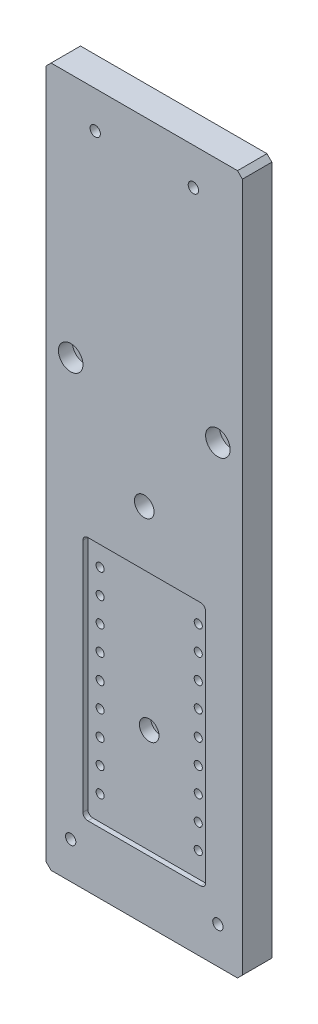
SolidWorks part; units mm, degrees
material "A6061"
ref_plane "前基準面" through (0, 0, 0) normal (0, 0, 1) x (1, 0, 0)
ref_plane "上基準面" through (0, 0, 0) normal (0, 1, 0) x (1, 0, 0)
ref_plane "右基準面" through (0, 0, 0) normal (1, 0, 0) x (0, 0, -1)
sketch "草图1" plane through (0, 0, 0) normal (0, 0, 1) x (1, 0, 0)
  line L1 (-40, 142.5) -> (40, 142.5)
  line L3 (-40, -142.5) -> (40, -142.5)
  line L4 (40, 142.5) -> (40, -142.5)
  line L5 (0, 0) -> (0, -119.2383) construction
  line L6 (0, 0) -> (187.1553, 0) construction
  line L8 (-40, 142.5) -> (-40, -142.5)
  dimension "D1" = 285
  dimension "D2" = 80
extrude "凸台-拉伸1" add sketch "草图1" along normal blind 12
hole_wizard "打孔尺寸(%根据)内六角圆柱头螺钉的类型1" positions "草图3" profile "草图4" counterbore size "M5" standard "GB" end condition up to next
sketch "草图3" plane through (0, 0, 12) normal (0, 0, 1) x (1, 0, 0)
  line L4 (0, 0) -> (0, -18.3877) construction
  line L8 (40, 142.5) -> (-40, 142.5) construction
  point P28 (-30, 42.5)
  point P53 (30, 42.5)
  dimension "D1" = 100
  dimension "D4" = 60
sketch "草图4" plane through (30, 42.5, 12) normal (1, 0, 0) x (0, -1, 0)
  line L0 (0, 0) -> (0, 12)
  line L1 (0, 12) -> (2.75, 12)
  line L3 (2.75, 12) -> (2.75, 5.7)
  line L4 (2.75, 5.7) -> (5, 5.7)
  line L5 (5, 5.7) -> (5, 0)
  line L7 (5, 0) -> (0, 0)
  line L11 (0, -6.35) -> (0, 107.95) construction
  dimension "通孔孔直径" = 5.5
  dimension "通孔孔深度" = 12
  dimension "柱形沉头孔直径" = 10
  dimension "柱形沉头孔深度" = 5.7
hole_wizard "M5 螺纹孔1" positions "草图23" profile "草图24" tap size "M5" standard "GB" end condition through all
sketch "草图23" plane through (0, 0, 0) normal (0, 0, -1) x (-1, 0, 0)
  line L0 (0, 227.7989) -> (0, 0) construction
  line L2 (-40, 142.5) -> (40, 142.5) construction
  point P0 (-20, 127.5)
  point P7 (20, 127.5)
  dimension "D1" = 40
  dimension "D2" = 15
sketch "草图24" plane through (20, 127.5, 0) normal (1, 0, 0) x (0, 1, 0)
  line L0 (0, 0) -> (0, 12)
  line L1 (0, 12) -> (2.1, 12)
  line L2 (2.1, 12) -> (2.1, 0)
  line L5 (2.1, 0) -> (0, 0)
  line L11 (0, -6.35) -> (0, 107.95) construction
  dimension "通孔螺纹孔钻头直径" = 4.2
  dimension "通孔螺纹孔钻头深度" = 12
cosmetic thread "孔螺蚊线1"
cosmetic thread "孔螺蚊线2"
sketch "草图25" plane through (0, 0, 12) normal (0, 0, 1) x (1, 0, 0)
  line L0 (0, 142.5) -> (0, -17.5) construction
  line L1 (-23, -17.5) -> (23, -17.5)
  line L2 (-25, -19.5) -> (-25, -115.5)
  line L3 (-23, -117.5) -> (23, -117.5)
  line L4 (25, -19.5) -> (25, -115.5)
  line L5 (40, 142.5) -> (-40, 142.5) construction
  line L6 (-40, -142.5) -> (40, -142.5) construction
  arc A0 (23, -117.5) -> (25, -115.5) centre (23, -115.5) ccw
  arc A1 (-25, -115.5) -> (-23, -117.5) centre (-23, -115.5) ccw
  arc A2 (-23, -17.5) -> (-25, -19.5) centre (-23, -19.5) ccw
  arc A3 (23, -17.5) -> (25, -19.5) centre (23, -19.5) cw
  dimension "D2" = 2
  dimension "D1" = 50
  dimension "D3" = 100
  dimension "D4" = 25
extrude "切除-拉伸2" cut sketch "草图25" against normal blind 2
hole_wizard "M4 螺纹孔1" positions "草图26" profile "草图27" tap size "M4" standard "GB" end condition through all
sketch "草图26" plane through (0, 0, 10) normal (0, 0, 1) x (1, 0, 0)
  line L0 (0, -17.5) -> (0, -117.5) construction
  line L1 (23, -17.5) -> (-23, -17.5) construction
  line L2 (-23, -117.5) -> (23, -117.5) construction
  line L4 (0, -67.5) -> (-40, -67.5) construction
  point P0 (-20, -27.5)
  point P4 (20, -27.5)
  point P5 (20, -37.5)
  point P6 (20, -47.5)
  point P7 (-20, -37.5)
  point P8 (-20, -47.5)
  point P19 (-20, -57.5)
  point P20 (20, -57.5)
  point P21 (-20, -67.5)
  point P22 (20, -67.5)
  point P23 (-20, -77.5)
  point P24 (20, -77.5)
  point P25 (-20, -87.5)
  point P26 (20, -87.5)
  point P27 (-20, -97.5)
  point P28 (20, -97.5)
  point P33 (-20, -107.5)
  point P34 (20, -107.5)
  dimension "D1" = 2
  dimension "D3" = 20
  dimension "D4" = 10
  dimension "D2" = 9
sketch "草图27" plane through (-20, -27.5, 10) normal (1, 0, 0) x (0, -1, 0)
  line L0 (0, 0) -> (0, 10)
  line L1 (0, 10) -> (1.65, 10)
  line L2 (1.65, 10) -> (1.65, 0)
  line L5 (1.65, 0) -> (0, 0)
  line L11 (0, -6.35) -> (0, 107.95) construction
  dimension "通孔螺纹孔钻头直径" = 3.3
  dimension "通孔螺纹孔钻头深度" = 10
cosmetic thread "孔螺蚊线3"
cosmetic thread "孔螺蚊线4"
cosmetic thread "孔螺蚊线5"
cosmetic thread "孔螺蚊线6"
cosmetic thread "孔螺蚊线7"
cosmetic thread "孔螺蚊线8"
cosmetic thread "孔螺蚊线9"
cosmetic thread "孔螺蚊线10"
cosmetic thread "孔螺蚊线11"
cosmetic thread "孔螺蚊线12"
cosmetic thread "孔螺蚊线15"
cosmetic thread "孔螺蚊线16"
cosmetic thread "孔螺蚊线17"
cosmetic thread "孔螺蚊线18"
cosmetic thread "孔螺蚊线19"
cosmetic thread "孔螺蚊线20"
cosmetic thread "孔螺蚊线21"
cosmetic thread "孔螺蚊线22"
hole_wizard "M5 螺纹孔2" positions "草图28" profile "草图29" tap size "M5" standard "GB" end condition through all
sketch "草图28" plane through (0, 0, 12) normal (0, 0, 1) x (1, 0, 0)
  line L0 (-40, -142.5) -> (40, -142.5) construction
  line L1 (0, 0) -> (0, -48.5506) construction
  point P0 (-30, -127.5)
  point P2 (30, -127.5)
  dimension "D1" = 60
  dimension "D2" = 15
sketch "草图29" plane through (-30, -127.5, 12) normal (1, 0, 0) x (0, -1, 0)
  line L0 (0, 0) -> (0, 12)
  line L1 (0, 12) -> (2.1, 12)
  line L2 (2.1, 12) -> (2.1, 0)
  line L5 (2.1, 0) -> (0, 0)
  line L11 (0, -6.35) -> (0, 107.95) construction
  dimension "通孔螺纹孔钻头直径" = 4.2
  dimension "通孔螺纹孔钻头深度" = 12
cosmetic thread "孔螺蚊线13"
cosmetic thread "孔螺蚊线14"
chamfer "倒角2" distance 2 angle 45 4 edges at (40, 142.5, 6) (40, -142.5, 6) (-40, -142.5, 6) (-40, 142.5, 6)
hole_wizard "打孔尺寸(%根据)内六角圆柱头螺钉的类型2" positions "草图30" profile "草图31" counterbore size "M4" standard "GB" end condition through all
sketch "草图30" plane through (0, 0, 12) normal (0, 0, 1) x (1, 0, 0)
  line L0 (-38, -142.5) -> (38, -142.5) construction
  point P0 (0, 5)
  point P2 (0, -75)
  dimension "D1" = 80
  dimension "D2" = 67.5
sketch "草图31" plane through (0, 5, 12) normal (1, 0, 0) x (0, -1, 0)
  line L0 (0, 0) -> (0, 12)
  line L1 (0, 12) -> (2.25, 12)
  line L3 (2.25, 12) -> (2.25, 6.6)
  line L4 (2.25, 6.6) -> (4, 6.6)
  line L5 (4, 6.6) -> (4, 0)
  line L7 (4, 0) -> (0, 0)
  line L11 (0, -6.35) -> (0, 107.95) construction
  dimension "通孔孔直径" = 4.5
  dimension "通孔孔深度" = 12
  dimension "柱形沉头孔直径" = 8
  dimension "柱形沉头孔深度" = 6.6
